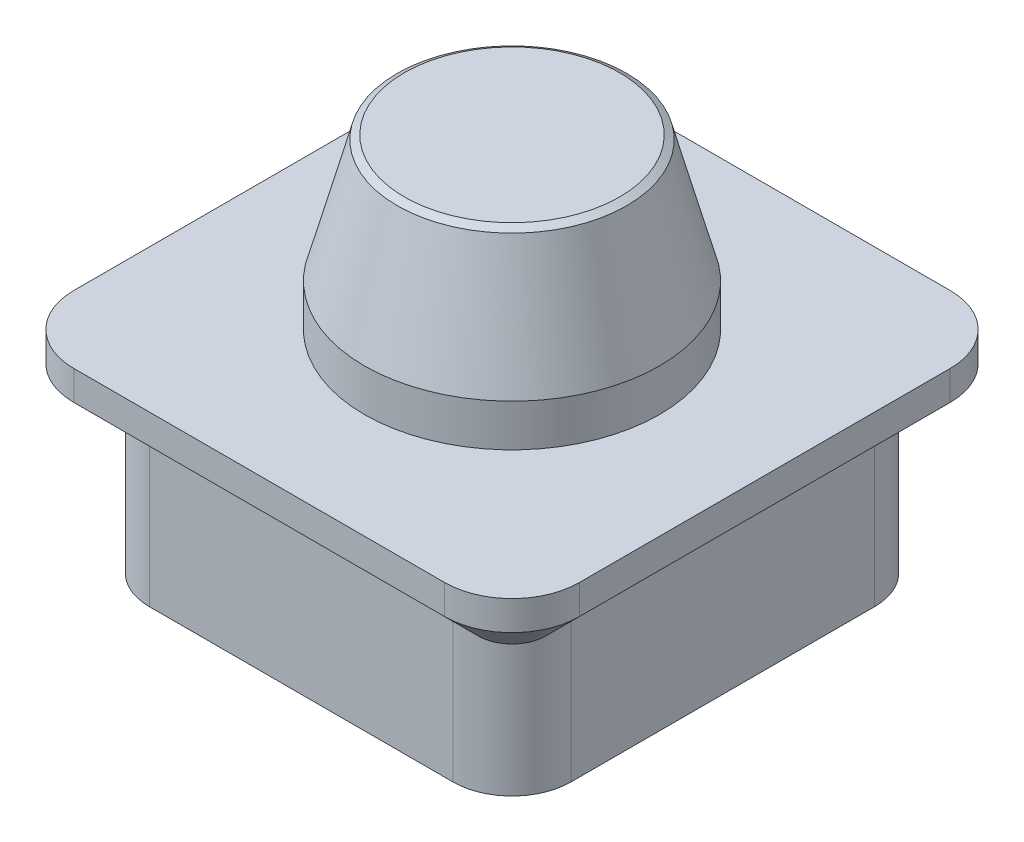
SolidWorks part; units mm, degrees
material "XRAAT"
ref_plane "前视基准面" through (0, 0, 0) normal (0, 0, 1) x (1, 0, 0)
ref_plane "上视基准面" through (0, 0, 0) normal (0, 1, 0) x (1, 0, 0)
ref_plane "右视基准面" through (0, 0, 0) normal (1, 0, 0) x (0, 0, -1)
sketch "草图1" plane through (0, 0, 0) normal (0, 0, 1) x (1, 0, 0)
  line L0 (0, 0) -> (35, 0)
  line L1 (35, 0) -> (35, 10)
  line L2 (35, 10) -> (26.9615, 40)
  line L3 (26.9615, 40) -> (0, 40)
  line L4 (0, 40) -> (0, -18.6749) construction
  line L5 (0, 0) -> (0, 40)
  dimension "D1" = 70
  dimension "D2" = 15
  dimension "D3" = 10
  dimension "D4" = 40
revolve "旋转1" add sketch "草图1" angle 360 about L4
chamfer "倒角1" distance 1 angle 45 1 edges at (-26.9615, 40, 0)
sketch "草图2" plane through (0, 0, 0) normal (0, -1, 0) x (1, 0, 0)
  line L1 (44, -60) -> (-44, -60)
  line L2 (60, -44) -> (60, 44)
  line L3 (44, 60) -> (-44, 60)
  line L4 (-60, -44) -> (-60, 44)
  line L5 (60, -60) -> (-60, 60) construction
  line L6 (60, 60) -> (-60, -60) construction
  arc A0 (-44, -60) -> (-60, -44) centre (-44, -44) cw
  arc A1 (60, 44) -> (44, 60) centre (44, 44) ccw
  arc A2 (44, -60) -> (60, -44) centre (44, -44) ccw
  arc A3 (-44, 60) -> (-60, 44) centre (-44, 44) ccw
  point P0 (0, 0)
  dimension "D2" = 16
  dimension "D1" = 120
extrude "凸台-拉伸1" add sketch "草图2" along normal blind 15
sketch "草图3" plane through (0, -15, 0) normal (0, -1, 0) x (1, 0, 0)
  line L1 (36, -50) -> (-36, -50)
  line L2 (50, -36) -> (50, 36)
  line L3 (36, 50) -> (-36, 50)
  line L4 (-50, -36) -> (-50, 36)
  line L5 (50, -50) -> (-50, 50) construction
  line L6 (50, 50) -> (-50, -50) construction
  arc A0 (-36, -50) -> (-50, -36) centre (-36, -36) cw
  arc A1 (50, 36) -> (36, 50) centre (36, 36) ccw
  arc A2 (36, -50) -> (50, -36) centre (36, -36) ccw
  arc A3 (-36, 50) -> (-50, 36) centre (-36, 36) ccw
  point P0 (0, 0)
  dimension "D2" = 14
  dimension "D1" = 100
extrude "凸台-拉伸2" add sketch "草图3" along normal blind 35
chamfer "倒角2" distance 8 angle 45 8 edges at (-55.3137, -15, -55.3137) (0, -15, -60) (-60, -15, 0) (55.3137, -15, -55.3137) (-55.3137, -15, 55.3137) (60, -15, 0) (0, -15, 60) (55.3137, -15, 55.3137)
